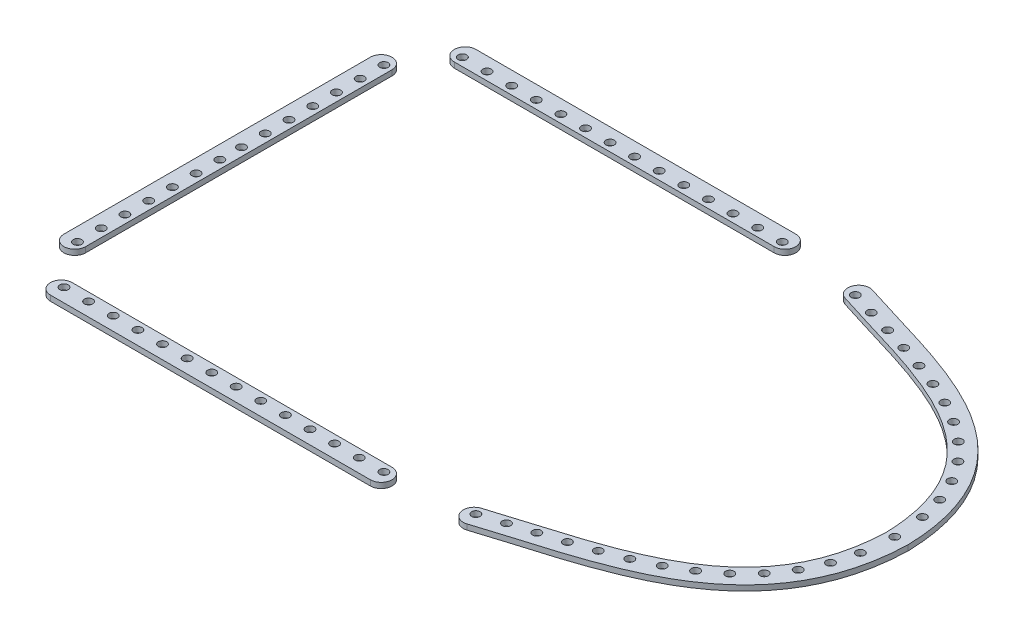
from build123d import *

# Parameters (mm, degrees)
SKETCH_1_R        = 1.55
EXTRUDE_1_DEPTH   = 2
EXTRUDE_1_2_DEPTH = 2
EXTRUDE_1_3_DEPTH = 2
EXTRUDE_1_4_DEPTH = 2


with BuildPart() as part:
    # 草图1 → 凸台-拉伸1 (new body)
    with BuildSketch(Plane(origin=(0, 0, 0), x_dir=(1, 0, 0), z_dir=(0, 1, 0))):
        with BuildLine():
            Line((56.529437252, -70.5), (-61.5, -70.5))
            ThreePointArc((-61.5, -70.5), (-65.5, -74.5), (-61.5, -78.5))
            Line((-61.5, -78.5), (56.529437252, -78.5))
            ThreePointArc((56.529437252, -78.5), (60.529437252, -74.5), (56.529437252, -70.5))
        make_face()
        with Locations(Location((56.529437252, -73.5, 0), (0, 0, 270))):
            Circle(SKETCH_1_R, mode=Mode.SUBTRACT)
        with Locations(Location((47.443650814, -73.5, 0), (0, 0, 270))):
            Circle(SKETCH_1_R, mode=Mode.SUBTRACT)
        with Locations(Location((38.357864376, -73.5, 0), (0, 0, 270))):
            Circle(SKETCH_1_R, mode=Mode.SUBTRACT)
        with Locations(Location((29.272077939, -73.5, 0), (0, 0, 270))):
            Circle(SKETCH_1_R, mode=Mode.SUBTRACT)
        with Locations(Location((20.186291501, -73.5, 0), (0, 0, 270))):
            Circle(SKETCH_1_R, mode=Mode.SUBTRACT)
        with Locations(Location((11.100505063, -73.5, 0), (0, 0, 270))):
            Circle(SKETCH_1_R, mode=Mode.SUBTRACT)
        with Locations(Location((2.014718626, -73.5, 0), (0, 0, 270))):
            Circle(SKETCH_1_R, mode=Mode.SUBTRACT)
        with Locations(Location((-6.985281374, -73.5, 0), (0, 0, 90))):
            Circle(SKETCH_1_R, mode=Mode.SUBTRACT)
        with Locations(Location((-16.071067812, -73.5, 0), (0, 0, 90))):
            Circle(SKETCH_1_R, mode=Mode.SUBTRACT)
        with Locations(Location((-25.156854249, -73.5, 0), (0, 0, 90))):
            Circle(SKETCH_1_R, mode=Mode.SUBTRACT)
        with Locations(Location((-34.242640687, -73.5, 0), (0, 0, 90))):
            Circle(SKETCH_1_R, mode=Mode.SUBTRACT)
        with Locations(Location((-43.328427125, -73.5, 0), (0, 0, 90))):
            Circle(SKETCH_1_R, mode=Mode.SUBTRACT)
        with Locations(Location((-52.414213562, -73.5, 0), (0, 0, 90))):
            Circle(SKETCH_1_R, mode=Mode.SUBTRACT)
        with Locations(Location((-61.5, -73.5, 0), (0, 0, 90))):
            Circle(SKETCH_1_R, mode=Mode.SUBTRACT)
    extrude(amount=EXTRUDE_1_DEPTH)


with BuildPart() as body_2:
    # 草图1 → Extrude 1 2 (new body)
    with BuildSketch(Plane(origin=(0, 0, 0), x_dir=(1, 0, 0), z_dir=(0, 1, 0))):
        with BuildLine():
            Line((-78.5, 56.529437252), (-78.5, -56.529437252))
            ThreePointArc((-78.5, -56.529437252), (-74.5, -60.529437252), (-70.5, -56.529437252))
            Line((-70.5, -56.529437252), (-70.5, 56.529437252))
            ThreePointArc((-70.5, 56.529437252), (-74.5, 60.529437252), (-78.5, 56.529437252))
        make_face()
        with Locations(Location((-73.5, -56.529437252, 0), (0, 0, 270))):
            Circle(SKETCH_1_R, mode=Mode.SUBTRACT)
        with Locations(Location((-73.5, -47.774531043, 0), (0, 0, 270))):
            Circle(SKETCH_1_R, mode=Mode.SUBTRACT)
        with Locations(Location((-73.5, -39.019624834, 0), (0, 0, 270))):
            Circle(SKETCH_1_R, mode=Mode.SUBTRACT)
        with Locations(Location((-73.5, -30.264718626, 0), (0, 0, 270))):
            Circle(SKETCH_1_R, mode=Mode.SUBTRACT)
        with Locations(Location((-73.5, -21.509812417, 0), (0, 0, 270))):
            Circle(SKETCH_1_R, mode=Mode.SUBTRACT)
        with Locations(Location((-73.5, -12.754906209, 0), (0, 0, 270))):
            Circle(SKETCH_1_R, mode=Mode.SUBTRACT)
        with Locations(Location((-73.5, -4, 0), (0, 0, 270))):
            Circle(SKETCH_1_R, mode=Mode.SUBTRACT)
        with Locations(Location((-73.5, 4, 0), (0, 0, 90))):
            Circle(SKETCH_1_R, mode=Mode.SUBTRACT)
        with Locations(Location((-73.5, 12.754906209, 0), (0, 0, 90))):
            Circle(SKETCH_1_R, mode=Mode.SUBTRACT)
        with Locations(Location((-73.5, 21.509812417, 0), (0, 0, 90))):
            Circle(SKETCH_1_R, mode=Mode.SUBTRACT)
        with Locations(Location((-73.5, 30.264718626, 0), (0, 0, 90))):
            Circle(SKETCH_1_R, mode=Mode.SUBTRACT)
        with Locations(Location((-73.5, 39.019624834, 0), (0, 0, 90))):
            Circle(SKETCH_1_R, mode=Mode.SUBTRACT)
        with Locations(Location((-73.5, 47.774531043, 0), (0, 0, 90))):
            Circle(SKETCH_1_R, mode=Mode.SUBTRACT)
        with Locations(Location((-73.5, 56.529437252, 0), (0, 0, 90))):
            Circle(SKETCH_1_R, mode=Mode.SUBTRACT)
    extrude(amount=EXTRUDE_1_2_DEPTH)


with BuildPart() as body_3:
    # 草图1 → Extrude 1 3 (new body)
    with BuildSketch(Plane(origin=(0, 0, 0), x_dir=(1, 0, 0), z_dir=(0, 1, 0))):
        with BuildLine():
            Line((56.529437252, 78.5), (-61.5, 78.5))
            ThreePointArc((-61.5, 78.5), (-65.5, 74.5), (-61.5, 70.5))
            Line((-61.5, 70.5), (56.529437252, 70.5))
            ThreePointArc((56.529437252, 70.5), (60.529437252, 74.5), (56.529437252, 78.5))
        make_face()
        with Locations(Location((-61.5, 73.5, 0), (0, 0, 270))):
            Circle(SKETCH_1_R, mode=Mode.SUBTRACT)
        with Locations(Location((-52.414213562, 73.5, 0), (0, 0, 270))):
            Circle(SKETCH_1_R, mode=Mode.SUBTRACT)
        with Locations(Location((-43.328427125, 73.5, 0), (0, 0, 270))):
            Circle(SKETCH_1_R, mode=Mode.SUBTRACT)
        with Locations(Location((-34.242640687, 73.5, 0), (0, 0, 270))):
            Circle(SKETCH_1_R, mode=Mode.SUBTRACT)
        with Locations(Location((-25.156854249, 73.5, 0), (0, 0, 270))):
            Circle(SKETCH_1_R, mode=Mode.SUBTRACT)
        with Locations(Location((-16.071067812, 73.5, 0), (0, 0, 270))):
            Circle(SKETCH_1_R, mode=Mode.SUBTRACT)
        with Locations(Location((-6.985281374, 73.5, 0), (0, 0, 270))):
            Circle(SKETCH_1_R, mode=Mode.SUBTRACT)
        with Locations(Location((2.014718626, 73.5, 0), (0, 0, 90))):
            Circle(SKETCH_1_R, mode=Mode.SUBTRACT)
        with Locations(Location((11.100505063, 73.5, 0), (0, 0, 90))):
            Circle(SKETCH_1_R, mode=Mode.SUBTRACT)
        with Locations(Location((20.186291501, 73.5, 0), (0, 0, 90))):
            Circle(SKETCH_1_R, mode=Mode.SUBTRACT)
        with Locations(Location((29.272077939, 73.5, 0), (0, 0, 90))):
            Circle(SKETCH_1_R, mode=Mode.SUBTRACT)
        with Locations(Location((38.357864376, 73.5, 0), (0, 0, 90))):
            Circle(SKETCH_1_R, mode=Mode.SUBTRACT)
        with Locations(Location((47.443650814, 73.5, 0), (0, 0, 90))):
            Circle(SKETCH_1_R, mode=Mode.SUBTRACT)
        with Locations(Location((56.529437252, 73.5, 0), (0, 0, 90))):
            Circle(SKETCH_1_R, mode=Mode.SUBTRACT)
    extrude(amount=EXTRUDE_1_3_DEPTH)


with BuildPart() as body_4:
    # 草图1 → Extrude 1 4 (new body)
    with BuildSketch(Plane(origin=(0, 0, 0), x_dir=(1, 0, 0), z_dir=(0, 1, 0))):
        with BuildLine():
            ThreePointArc((86.032612563, 67.150394861), (83.483739291, 72.200468627), (88.533813058, 74.749341899))
            add(Edge.make_bspline(
                [(176.502121182, 0), (176.477673441, 0.839215895), (176.408789589, 2.528107014), (176.171608814, 5.812988702), (175.701085249, 9.7769902), (174.862637139, 14.302752959), (173.392140428, 20.038350433), (170.915409862, 26.655034839), (167.014299419, 33.731777805), (162.301605231, 39.97128723), (155.107874482, 47.238684399), (144.733534828, 54.524687611), (130.930997657, 61.106504363), (118.882288587, 65.386235026), (109.251922463, 68.407626718), (102.117197123, 70.547995844), (96.324722793, 72.285245719), (91.812493453, 73.686740135), (89.630650754, 74.388316749), (88.533813058, 74.749341899)],
                knots=[-0.00094592, -0.00094592, -0.00094592, -0.00094592, 0.01469386, 0.03033364, 0.0616132, 0.09289276, 0.12417232, 0.18673144, 0.24929056, 0.31184968, 0.3744088, 0.49952704, 0.62464528, 0.74976352, 0.81232264, 0.87488176, 0.93744088, 0.96872044, 1, 1, 1, 1], degree=3))
            add(Edge.make_bspline(
                [(88.533813058, -74.749341899), (89.630650754, -74.388316749), (91.812493453, -73.686740135), (96.324722793, -72.285245719), (102.117197123, -70.547995844), (109.251922463, -68.407626718), (118.882288587, -65.386235026), (130.930997657, -61.106504363), (144.733534828, -54.524687611), (155.107874482, -47.238684399), (162.301605231, -39.97128723), (167.014299419, -33.731777805), (170.915409862, -26.655034839), (173.392140428, -20.038350433), (174.862637139, -14.302752959), (175.701085249, -9.7769902), (176.171608814, -5.812988702), (176.408789589, -2.528107014), (176.477673441, -0.839215895), (176.502121182, 0)],
                knots=[-0.00094592, -0.00094592, -0.00094592, -0.00094592, 0.03033364, 0.0616132, 0.12417232, 0.18673144, 0.24929056, 0.3744088, 0.49952704, 0.62464528, 0.6872044, 0.74976352, 0.81232264, 0.87488176, 0.90616132, 0.93744088, 0.96872044, 0.98436022, 1, 1, 1, 1], degree=3))
            ThreePointArc((88.533813058, -74.749341899), (83.483739291, -72.200468627), (86.032612563, -67.150394861))
            add(Edge.make_bspline(
                [(168.498679683, 0), (168.47568853, -0.760741418), (168.406948846, -2.296877119), (168.186204793, -5.241976411), (167.755474322, -8.77444778), (167.004163495, -12.758988425), (165.705489153, -17.757623571), (163.554482879, -23.443053135), (160.210118817, -29.468324372), (156.168954452, -34.794459554), (149.931240351, -41.077560259), (140.689680327, -47.578033775), (127.871224852, -53.699621041), (116.3130299, -57.808108695), (106.887704501, -60.764606755), (99.813650665, -62.886822441), (93.988849474, -64.633767009), (89.403347408, -66.057958815), (87.157830193, -66.78002843), (86.032612563, -67.150394861)],
                knots=[0.000589076, 0.000589076, 0.000589076, 0.000589076, 0.016204871, 0.031820667, 0.063052258, 0.09428385, 0.125515441, 0.187978624, 0.250441807, 0.312904989, 0.375368172, 0.500294538, 0.625220903, 0.750147269, 0.812610452, 0.875073634, 0.937536817, 0.968768409, 1, 1, 1, 1], degree=3))
            add(Edge.make_bspline(
                [(86.032612563, 67.150394861), (87.157830193, 66.78002843), (89.403347408, 66.057958815), (93.988849474, 64.633767009), (99.813650665, 62.886822441), (106.887704501, 60.764606755), (116.3130299, 57.808108695), (127.871224852, 53.699621041), (140.689680327, 47.578033775), (149.931240351, 41.077560259), (156.168954452, 34.794459554), (160.210118817, 29.468324372), (163.554482879, 23.443053135), (165.705489153, 17.757623571), (167.004163495, 12.758988425), (167.755474322, 8.77444778), (168.186204793, 5.241976411), (168.406948846, 2.296877119), (168.47568853, 0.760741418), (168.498679683, 0)],
                knots=[0.000589076, 0.000589076, 0.000589076, 0.000589076, 0.031820667, 0.063052258, 0.125515441, 0.187978624, 0.250441807, 0.375368172, 0.500294538, 0.625220903, 0.687684086, 0.750147269, 0.812610452, 0.875073634, 0.906305226, 0.937536817, 0.968768409, 0.984384204, 1, 1, 1, 1], degree=3))
        make_face()
        with Locations(Location((86.970562748, 70, 0), (0, 0, 270))):
            Circle(SKETCH_1_R, mode=Mode.SUBTRACT)
        with Locations(Location((95.556662166, 67.302056933, 0), (0, 0, 270))):
            Circle(SKETCH_1_R, mode=Mode.SUBTRACT)
        with Locations(Location((104.174893516, 64.708586593, 0), (0, 0, 270))):
            Circle(SKETCH_1_R, mode=Mode.SUBTRACT)
        with Locations(Location((112.773503296, 62.0507849, 0), (0, 0, 270))):
            Circle(SKETCH_1_R, mode=Mode.SUBTRACT)
        with Locations(Location((121.301072962, 59.173189445, 0), (0, 0, 270))):
            Circle(SKETCH_1_R, mode=Mode.SUBTRACT)
        with Locations(Location((129.691902577, 55.918350223, 0), (0, 0, 270))):
            Circle(SKETCH_1_R, mode=Mode.SUBTRACT)
        with Locations(Location((137.84994583, 52.117517382, 0), (0, 0, 270))):
            Circle(SKETCH_1_R, mode=Mode.SUBTRACT)
        with Locations(Location((145.628708479, 47.590835192, 0), (0, 0, 270))):
            Circle(SKETCH_1_R, mode=Mode.SUBTRACT)
        with Locations(Location((152.81108962, 42.167422876, 0), (0, 0, 270))):
            Circle(SKETCH_1_R, mode=Mode.SUBTRACT)
        with Locations(Location((159.109343971, 35.738426676, 0), (0, 0, 270))):
            Circle(SKETCH_1_R, mode=Mode.SUBTRACT)
        with Locations(Location((164.222345967, 28.331861306, 0), (0, 0, 270))):
            Circle(SKETCH_1_R, mode=Mode.SUBTRACT)
        with Locations(Location((167.952877754, 20.141431978, 0), (0, 0, 270))):
            Circle(SKETCH_1_R, mode=Mode.SUBTRACT)
        with Locations(Location((170.292118879, 11.450750131, 0), (0, 0, 270))):
            Circle(SKETCH_1_R, mode=Mode.SUBTRACT)
        with Locations(Location((171.5, 0, 0), (0, 0, 270))):
            Circle(SKETCH_1_R, mode=Mode.SUBTRACT)
        with Locations(Location((170.292118879, -11.450750131, 0), (0, 0, 90))):
            Circle(SKETCH_1_R, mode=Mode.SUBTRACT)
        with Locations(Location((167.952877754, -20.141431978, 0), (0, 0, 90))):
            Circle(SKETCH_1_R, mode=Mode.SUBTRACT)
        with Locations(Location((164.222345967, -28.331861306, 0), (0, 0, 90))):
            Circle(SKETCH_1_R, mode=Mode.SUBTRACT)
        with Locations(Location((159.109343971, -35.738426676, 0), (0, 0, 90))):
            Circle(SKETCH_1_R, mode=Mode.SUBTRACT)
        with Locations(Location((152.81108962, -42.167422876, 0), (0, 0, 90))):
            Circle(SKETCH_1_R, mode=Mode.SUBTRACT)
        with Locations(Location((145.628708479, -47.590835192, 0), (0, 0, 90))):
            Circle(SKETCH_1_R, mode=Mode.SUBTRACT)
        with Locations(Location((137.84994583, -52.117517382, 0), (0, 0, 90))):
            Circle(SKETCH_1_R, mode=Mode.SUBTRACT)
        with Locations(Location((129.691902577, -55.918350223, 0), (0, 0, 90))):
            Circle(SKETCH_1_R, mode=Mode.SUBTRACT)
        with Locations(Location((121.301072962, -59.173189445, 0), (0, 0, 90))):
            Circle(SKETCH_1_R, mode=Mode.SUBTRACT)
        with Locations(Location((112.773503296, -62.0507849, 0), (0, 0, 90))):
            Circle(SKETCH_1_R, mode=Mode.SUBTRACT)
        with Locations(Location((104.174893516, -64.708586593, 0), (0, 0, 90))):
            Circle(SKETCH_1_R, mode=Mode.SUBTRACT)
        with Locations(Location((95.556662166, -67.302056933, 0), (0, 0, 90))):
            Circle(SKETCH_1_R, mode=Mode.SUBTRACT)
        with Locations(Location((86.970562748, -70, 0), (0, 0, 90))):
            Circle(SKETCH_1_R, mode=Mode.SUBTRACT)
    extrude(amount=EXTRUDE_1_4_DEPTH)


solid = Compound([part.part, body_2.part, body_3.part, body_4.part])
